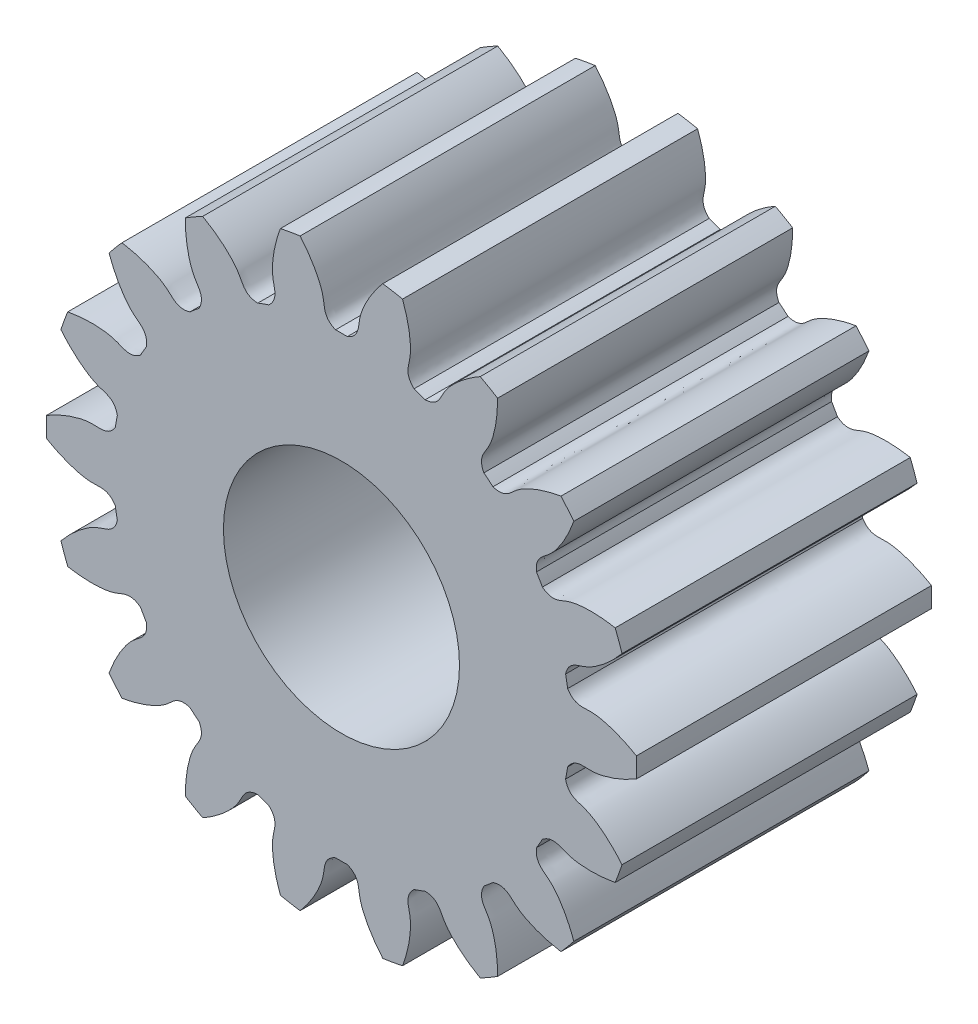
from build123d import *

# Parameters (mm, degrees)
SKETCH1_R           = 10
BOSS_EXTRUDE1_DEPTH = 10
CUT_EXTRUDE1_DEPTH  = 18.320508076
CIRPATTERN1_COUNT   = 18
SKETCH4_R           = 4
CUT_EXTRUDE2_DEPTH  = 18.263755653
CUT_EXTRUDE3_DEPTH  = 1.4


with BuildPart() as part:
    # Sketch1 → Boss-Extrude1 (new body)
    with BuildSketch(Plane.XY):
        Circle(SKETCH1_R)
    extrude(amount=BOSS_EXTRUDE1_DEPTH)

    # Sketch2 → Cut-Extrude1 (cut, through all)
    with BuildSketch(Plane.XY):
        with BuildLine():
            ThreePointArc((0.199403559, 7.747434299), (0, 7.75), (-0.199403559, 7.747434299))
            add(Edge.make_bspline(
                [(-0.199403559, 7.747434299), (-0.61510404, 7.918680391), (-0.56278905, 8.238699502), (-0.631832915, 8.542595456), (-0.63875152, 8.570506601), (-0.647107593, 8.601540475), (-0.65702471, 8.635650183), (-0.668630031, 8.672784168), (-0.682047718, 8.712887332), (-0.697400853, 8.755900732), (-0.714810717, 8.801761729), (-0.734396875, 8.850403997), (-0.756277026, 8.901757578), (-0.780566921, 8.955748932), (-0.807380259, 9.01230098), (-0.836828597, 9.071333165), (-0.869021256, 9.132761504), (-0.904065225, 9.196498643), (-0.942065076, 9.262453924), (-0.98312287, 9.330533439), (-1.027338072, 9.400640102), (-1.074807462, 9.472673712), (-1.125625055, 9.54653102), (-1.179882014, 9.622105805), (-1.237666571, 9.699288945), (-1.299063947, 9.777968491), (-1.364156275, 9.858029744), (-1.433022524, 9.939355337), (-1.505738425, 10.021825314), (-1.582376404, 10.105317214), (-1.663005502, 10.189706153), (-1.747691321, 10.274864914), (-1.836495946, 10.360664035), (-1.929477891, 10.446971896), (-2.026692033, 10.533654813), (-2.128189554, 10.620577131), (-2.234017887, 10.707601317), (-2.34422066, 10.79458806), (-2.45883764, 10.881396363), (-2.577904698, 10.967883646), (-2.701453724, 11.053905845), (-2.874075353, 11.169039516), (-3.007555439, 11.252333779), (-3.098560891, 11.30667838)],
                knots=[0, 0, 0, 0, 0.187591972, 0.192996016, 0.1991206, 0.205965723, 0.213531386, 0.221817587, 0.230824328, 0.240551609, 0.250999428, 0.262167787, 0.274056685, 0.286666122, 0.299996099, 0.314046614, 0.32881767, 0.344309264, 0.360521397, 0.37745407, 0.395107283, 0.413481034, 0.432575325, 0.452390155, 0.472925524, 0.494181432, 0.51615788, 0.538854867, 0.562272393, 0.586410459, 0.611269064, 0.636848208, 0.663147891, 0.690168114, 0.717908876, 0.746370177, 0.775552017, 0.805454397, 0.836077316, 0.867420774, 0.899484772, 0.932269309, 1, 1, 1, 1], degree=3))
            ThreePointArc((-3.098560891, 11.30667838), (0, 11.723568381), (3.098560891, 11.30667838))
            add(Edge.make_bspline(
                [(0.199403559, 7.747434299), (0.61510404, 7.918680391), (0.56278905, 8.238699502), (0.631832915, 8.542595456), (0.63875152, 8.570506601), (0.647107593, 8.601540475), (0.65702471, 8.635650183), (0.668630031, 8.672784168), (0.682047718, 8.712887332), (0.697400853, 8.755900732), (0.714810717, 8.801761729), (0.734396875, 8.850403997), (0.756277026, 8.901757578), (0.780566921, 8.955748932), (0.807380259, 9.01230098), (0.836828597, 9.071333165), (0.869021256, 9.132761504), (0.904065225, 9.196498643), (0.942065076, 9.262453924), (0.98312287, 9.330533439), (1.027338072, 9.400640102), (1.074807462, 9.472673712), (1.125625055, 9.54653102), (1.179882014, 9.622105805), (1.237666571, 9.699288945), (1.299063947, 9.777968491), (1.364156275, 9.858029744), (1.433022524, 9.939355337), (1.505738425, 10.021825314), (1.582376404, 10.105317214), (1.663005502, 10.189706153), (1.747691321, 10.274864914), (1.836495946, 10.360664035), (1.929477891, 10.446971896), (2.026692033, 10.533654813), (2.128189554, 10.620577131), (2.234017887, 10.707601317), (2.34422066, 10.79458806), (2.45883764, 10.881396363), (2.577904698, 10.967883646), (2.701453724, 11.053905845), (2.874075353, 11.169039516), (3.007555439, 11.252333779), (3.098560891, 11.30667838)],
                knots=[0, 0, 0, 0, 0.187591972, 0.192996016, 0.1991206, 0.205965723, 0.213531386, 0.221817587, 0.230824328, 0.240551609, 0.250999428, 0.262167787, 0.274056685, 0.286666122, 0.299996099, 0.314046614, 0.32881767, 0.344309264, 0.360521397, 0.37745407, 0.395107283, 0.413481034, 0.432575325, 0.452390155, 0.472925524, 0.494181432, 0.51615788, 0.538854867, 0.562272393, 0.586410459, 0.611269064, 0.636848208, 0.663147891, 0.690168114, 0.717908876, 0.746370177, 0.775552017, 0.805454397, 0.836077316, 0.867420774, 0.899484772, 0.932269309, 1, 1, 1, 1], degree=3))
        make_face()
    cut_extrude1 = extrude(amount=CUT_EXTRUDE1_DEPTH, mode=Mode.SUBTRACT)

    # CirPattern1: Cut-Extrude1 ×18 about axis
    cirpattern1_axis = Axis((0, 0, 10), (0, 0, -1))
    for i in range(1, CIRPATTERN1_COUNT):
        add(cut_extrude1.rotate(cirpattern1_axis, i * 360 / CIRPATTERN1_COUNT), mode=Mode.SUBTRACT)

    # Sketch4 → Cut-Extrude2 (cut, through all)
    with BuildSketch(Plane.XY.offset(10)):
        Circle(SKETCH4_R)
    extrude(amount=-CUT_EXTRUDE2_DEPTH, mode=Mode.SUBTRACT)

    # Sketch5 → Cut-Extrude3 (cut, symmetric)
    with BuildSketch(Plane(origin=(0, 4, 0), x_dir=(1, 0, 0), z_dir=(0, 1, 0))):
        with BuildLine():
            Line((1.5, -1.5), (1.5, -6.5))
            ThreePointArc((1.5, -6.5), (0, -8), (-1.5, -6.5))
            Line((-1.5, -6.5), (-1.5, -1.5))
            Line((-1.5, -1.5), (-1.5, 1.271150893))
            Line((-1.5, 1.271150893), (1.5, 1.271150893))
            Line((1.5, 1.271150893), (1.5, -1.5))
        make_face()
    extrude(amount=CUT_EXTRUDE3_DEPTH, both=True, mode=Mode.SUBTRACT)


solid = part.part
